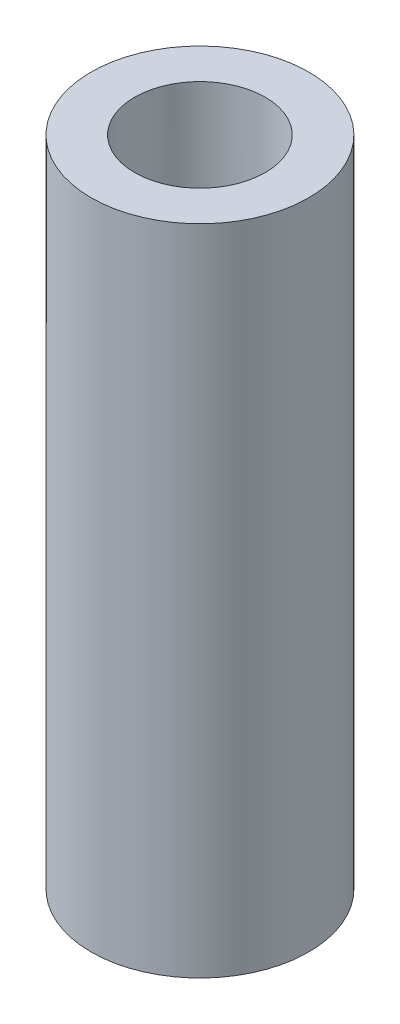
from build123d import *

# Parameters (mm, degrees)
SKETCH1_R           = 2.5
SKETCH1_R_2         = 1.5
BOSS_EXTRUDE1_DEPTH = 15
SKETCH2_R           = 1.5
SKETCH2_R_2         = 0.5
BOSS_EXTRUDE2_DEPTH = 2


with BuildPart() as part:
    # Sketch1 → Boss-Extrude1 (new body)
    with BuildSketch(Plane(origin=(0, 0, 0), x_dir=(1, 0, 0), z_dir=(0, 1, 0))):
        with Locations(Location((0, 0, 0), (0, 0, 270))):
            Circle(SKETCH1_R)
        with Locations(Location((0, 0, 0), (0, 0, 270))):
            Circle(SKETCH1_R_2, mode=Mode.SUBTRACT)
    extrude(amount=BOSS_EXTRUDE1_DEPTH)

    # Sketch2 → Boss-Extrude2 (add)
    with BuildSketch(Plane.XZ):
        with Locations(Location((0, 0, 0), (0, 0, 270))):
            Circle(SKETCH2_R)
        with Locations(Location((0, 0, 0), (0, 0, 270))):
            Circle(SKETCH2_R_2, mode=Mode.SUBTRACT)
    extrude(amount=-BOSS_EXTRUDE2_DEPTH)


solid = part.part
